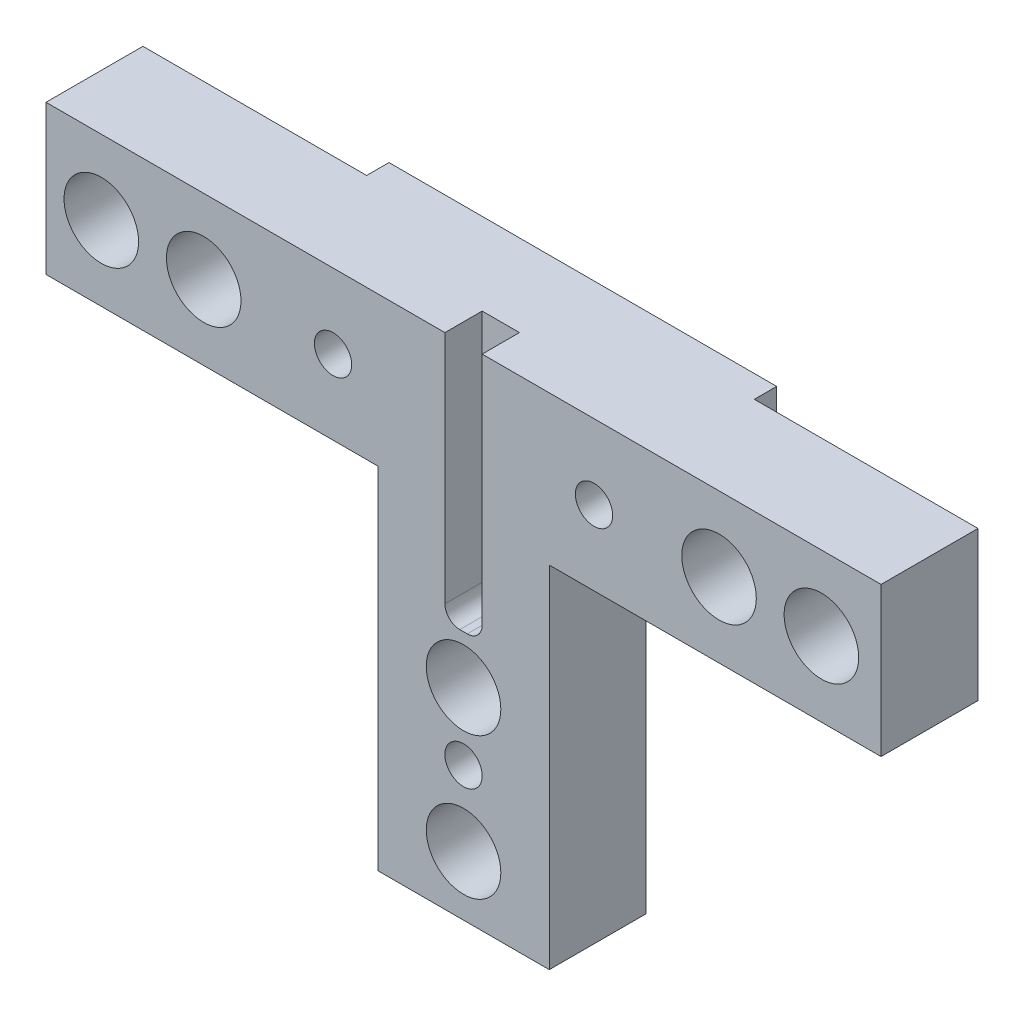
SolidWorks part; units mm, degrees
ref_plane "前视基准面" through (0, 0, 0) normal (0, 0, 1) x (1, 0, 0)
ref_plane "上视基准面" through (0, 0, 0) normal (0, 1, 0) x (1, 0, 0)
ref_plane "右视基准面" through (0, 0, 0) normal (1, 0, 0) x (0, 0, -1)
sketch "草图1" plane through (0, 0, 0) normal (0, 0, 1) x (1, 0, 0)
  line L0 (-47.8318, 24.7414) -> (64.1682, 24.7414)
  line L1 (64.1682, 24.7414) -> (64.1682, 4.7414)
  line L2 (64.1682, 4.7414) -> (19.6682, 4.7414)
  line L3 (19.6682, 4.7414) -> (19.6682, -42.2586)
  line L4 (19.6682, -42.2586) -> (-3.3318, -42.2586)
  line L5 (-3.3318, -42.2586) -> (-3.3318, 4.7414)
  line L6 (-3.3318, 4.7414) -> (-47.8318, 4.7414)
  line L7 (-47.8318, 4.7414) -> (-47.8318, 24.7414)
  dimension "D1" = 112
  dimension "D2" = 20
  dimension "D3" = 20
  dimension "D4" = 44.5
  dimension "D5" = 44.5
  dimension "D6" = 47
extrude "凸台-拉伸1" add sketch "草图1" along normal blind 16
sketch "草图2" plane through (0, 0, 0) normal (0, 0, -1) x (-1, 0, 0)
  line L0 (-19.6682, 4.7414) -> (-64.1682, 4.7414) construction
  line L1 (-64.1682, 24.7414) -> (-34.1682, 24.7414)
  line L2 (-64.1682, 24.7414) -> (-64.1682, 4.7414)
  line L3 (-64.1682, 4.7414) -> (-34.1682, 4.7414)
  line L4 (-34.1682, 24.7414) -> (-34.1682, 4.7414)
  line L5 (-19.6682, -42.2586) -> (-19.6682, 4.7414) construction
  line L6 (-19.6682, -7.2586) -> (3.3318, -7.2586)
  line L7 (-19.6682, -7.2586) -> (-19.6682, -42.2586)
  line L8 (-19.6682, -42.2586) -> (3.3318, -42.2586)
  line L9 (3.3318, -7.2586) -> (3.3318, -42.2586)
  line L10 (-64.1682, 24.7414) -> (47.8318, 24.7414) construction
  line L11 (17.8318, 24.7414) -> (47.8318, 24.7414)
  line L12 (17.8318, 24.7414) -> (17.8318, 4.7414)
  line L13 (17.8318, 4.7414) -> (47.8318, 4.7414)
  line L14 (47.8318, 24.7414) -> (47.8318, 4.7414)
  dimension "D1" = 30
  dimension "D2" = 30
  dimension "D3" = 35
extrude "切除-拉伸1" cut sketch "草图2" against normal blind 3
sketch "草图3" plane through (0, 0, 16) normal (0, 0, 1) x (1, 0, 0)
  line L0 (64.1682, 24.7414) -> (-47.8318, 24.7414) construction
  line L1 (10.6682, 24.7414) -> (5.6682, 24.7414)
  line L2 (10.6682, 24.7414) -> (10.6682, -6.7552)
  line L4 (5.6682, 24.7414) -> (5.6682, -6.7552)
  line L5 (-47.8318, 24.7414) -> (-47.8318, 4.7414) construction
  line L6 (8.6682, -8.7552) -> (7.6682, -8.7552)
  arc A0 (8.6682, -8.7552) -> (10.6682, -6.7552) centre (8.6682, -6.7552) ccw
  arc A1 (5.6682, -6.7552) -> (7.6682, -8.7552) centre (7.6682, -6.7552) ccw
  dimension "D3" = 4
  dimension "D4" = 4
  dimension "D1" = 5
  dimension "D2" = 53.5
extrude "切除-拉伸2" cut sketch "草图3" against normal blind 5
sketch "草图4" plane through (0, 0, 16) normal (0, 0, 1) x (1, 0, 0)
  line L0 (64.1682, 4.7414) -> (64.1682, 24.7414) construction
  line L1 (64.1682, 24.7414) -> (10.6682, 24.7414) construction
  circle A0 centre (56.1682, 14.7414) radius 2.75
  circle A1 centre (42.4352, 14.7414) radius 2.75
  circle A2 centre (-26.6818, 14.7414) radius 2.75
  circle A3 centre (-40.4148, 14.7414) radius 2.75
  dimension "D1" = 5.5
  dimension "D2" = 8
  dimension "D3" = 10
  dimension "D4" = 2
  dimension "D5" = 2
extrude "切除-拉伸3" cut sketch "草图4" against normal up to next
sketch "草图5" plane through (0, 0, 3) normal (0, 0, -1) x (-1, 0, 0)
  line L0 (-19.6682, -42.2586) -> (3.3318, -42.2586) construction
  line L1 (3.3318, -42.2586) -> (3.3318, -7.2586) construction
  circle A0 centre (-8.1682, -15.2586) radius 2.75
  circle A1 centre (-8.1682, -34.2586) radius 2.75
  dimension "D1" = 5.5
  dimension "D2" = 5.5
  dimension "D3" = 8
  dimension "D4" = 11.5
  dimension "D5" = 11.5
  dimension "D6" = 19
extrude "切除-拉伸4" cut sketch "草图5" against normal up to next
sketch "草图6" plane through (0, 0, 16) normal (0, 0, 1) x (1, 0, 0)
  circle A0 centre (-40.4148, 14.7414) radius 5
  circle A1 centre (-26.6818, 14.7414) radius 5
  circle A2 centre (42.4352, 14.7414) radius 5
  circle A3 centre (56.1682, 14.7414) radius 5
  circle A4 centre (8.1682, -15.2586) radius 5
  circle A5 centre (8.1682, -34.2586) radius 5
  dimension "D1" = 10
  dimension "D2" = 10
  dimension "D3" = 10
  dimension "D4" = 10
  dimension "D5" = 10
  dimension "D6" = 10
extrude "切除-拉伸5" cut sketch "草图6" against normal blind 9
sketch "草图7" plane through (0, 0, 16) normal (0, 0, 1) x (1, 0, 0)
  line L0 (64.1682, 24.7414) -> (10.6682, 24.7414) construction
  line L1 (10.6682, -6.7552) -> (10.6682, 24.7414) construction
  line L2 (8.1682, 24.7414) -> (8.1682, -49975.2586) construction
  line L3 (10.6682, 24.7414) -> (5.6682, 24.7414) construction
  line L5 (-3.3318, -42.2586) -> (19.6682, -42.2586) construction
  circle A1 centre (25.6682, 14.7414) radius 2.1
  circle A2 centre (-9.3318, 14.7414) radius 2.1
  circle A5 centre (8.1682, -24.2586) radius 2.1
  point P11 (8.1682, 24.7414)
  dimension "D2" = 4.2
  dimension "D6" = 4.2
  dimension "D3" = 10
  dimension "D4" = 15
  dimension "D7" = 18
extrude "切除-拉伸6" cut sketch "草图7" against normal blind 12.5
sketch "草图8" plane through (0, 0, 16) normal (0, 0, 1) x (1, 0, 0)
  circle A0 centre (-9.3318, 14.7414) radius 2.5
  circle A1 centre (25.6682, 14.7414) radius 2.5
  circle A2 centre (8.1682, -24.2586) radius 2.5
  dimension "D1" = 5
  dimension "D2" = 5
  dimension "D3" = 5
extrude "切除-拉伸7" cut sketch "草图8" against normal blind 10
